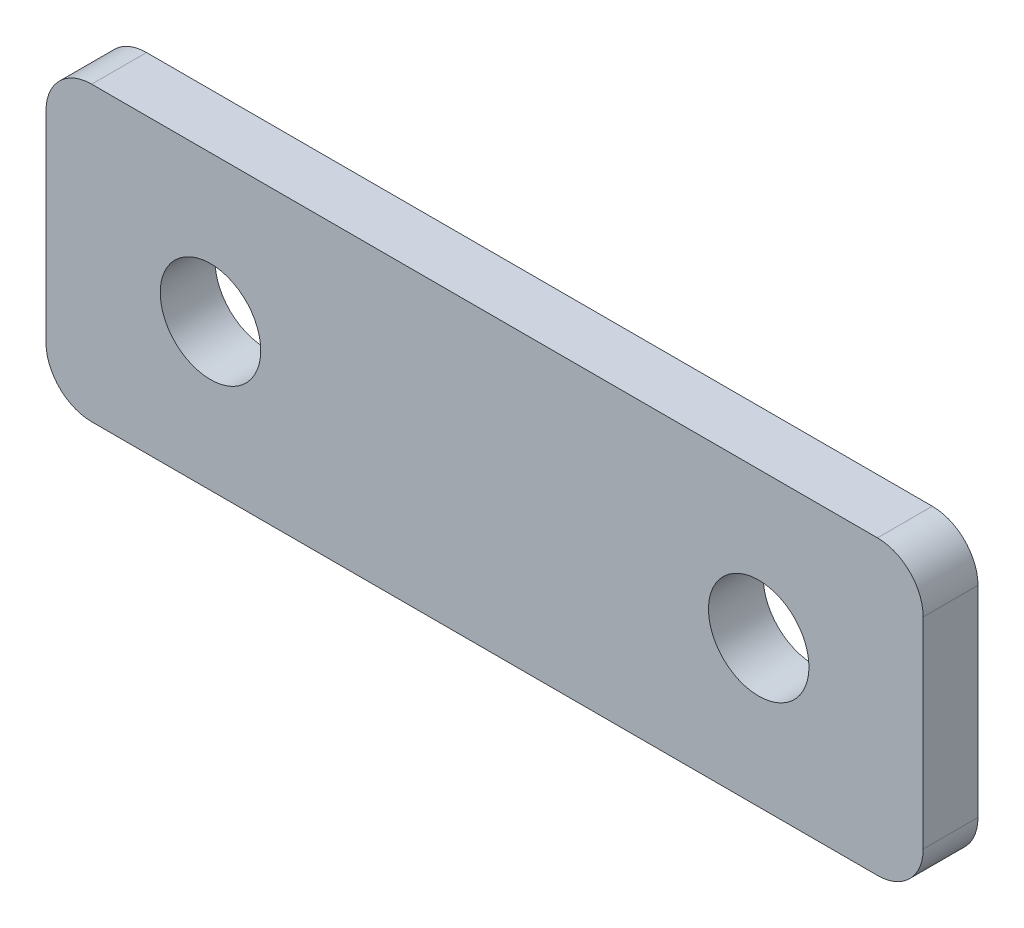
SolidWorks part; units mm, degrees
material "Plain Carbon Steel"
ref_plane "Front Plane" through (0, 0, 0) normal (0, 0, 1) x (1, 0, 0)
ref_plane "Top Plane" through (0, 0, 0) normal (0, 1, 0) x (1, 0, 0)
ref_plane "Right Plane" through (0, 0, 0) normal (1, 0, 0) x (0, 0, -1)
sketch "Sketch1" plane through (0, 0, 0) normal (0, 0, 1) x (1, 0, 0)
  line L1 (0, 0) -> (96, 0)
  line L2 (0, 0) -> (0, -32)
  line L3 (0, -32) -> (96, -32)
  line L4 (96, 0) -> (96, -32)
  dimension "D1" = 96
  dimension "D2" = 32
extrude "Boss-Extrude1" add sketch "Sketch1" along normal blind 6
fillet "Fillet1" radius 5 4 edges at (96, 0, 3) (96, -32, 3) (0, -32, 3) (0, 0, 3)
sketch "Sketch2" plane through (0, 0, 6) normal (0, 0, 1) x (1, 0, 0)
  line L0 (91, 0) -> (5, 0) construction
  line L1 (0, -5) -> (0, -27) construction
  circle A0 centre (18, -16) radius 5.5
  dimension "D3" = 11
  dimension "D1" = 16
  dimension "D2" = 18
extrude "Cut-Extrude1" cut sketch "Sketch2" against normal blind 6
pattern_linear "LPattern1" count 2 spacing 60 along (1, 0, 0) of "Cut-Extrude1"
